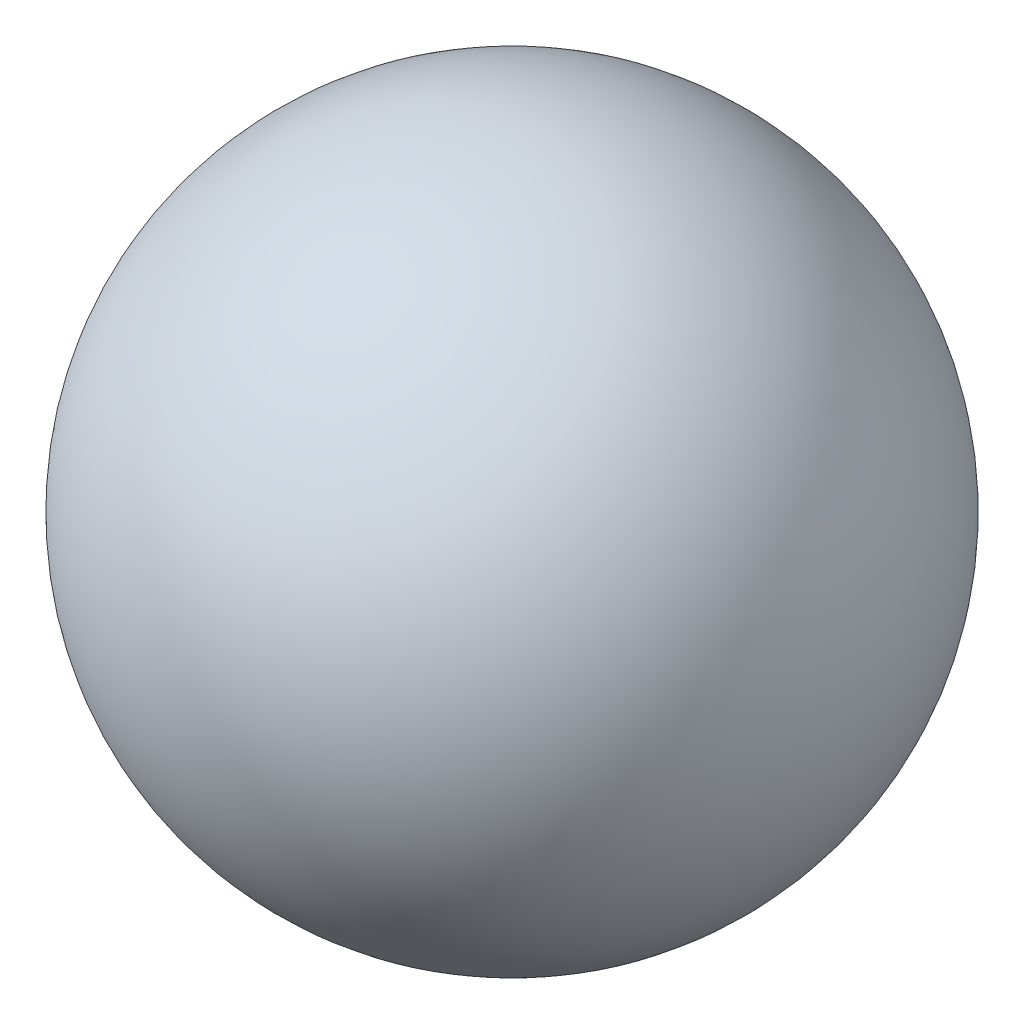
SolidWorks part; units mm, degrees
ref_plane "前视基准面" through (0, 0, 0) normal (0, 0, 1) x (1, 0, 0)
ref_plane "上视基准面" through (0, 0, 0) normal (0, 1, 0) x (1, 0, 0)
ref_plane "右视基准面" through (0, 0, 0) normal (1, 0, 0) x (0, 0, -1)
sketch "草图1" plane through (0, 0, 0) normal (0, 0, 1) x (1, 0, 0)
  line L0 (0, 50) -> (0, -50)
  arc A0 (0, -50) -> (0, 50) centre (0, 0) ccw
  dimension "D1" = 50
revolve "旋转1" add sketch "草图1" angle 360 about L0
